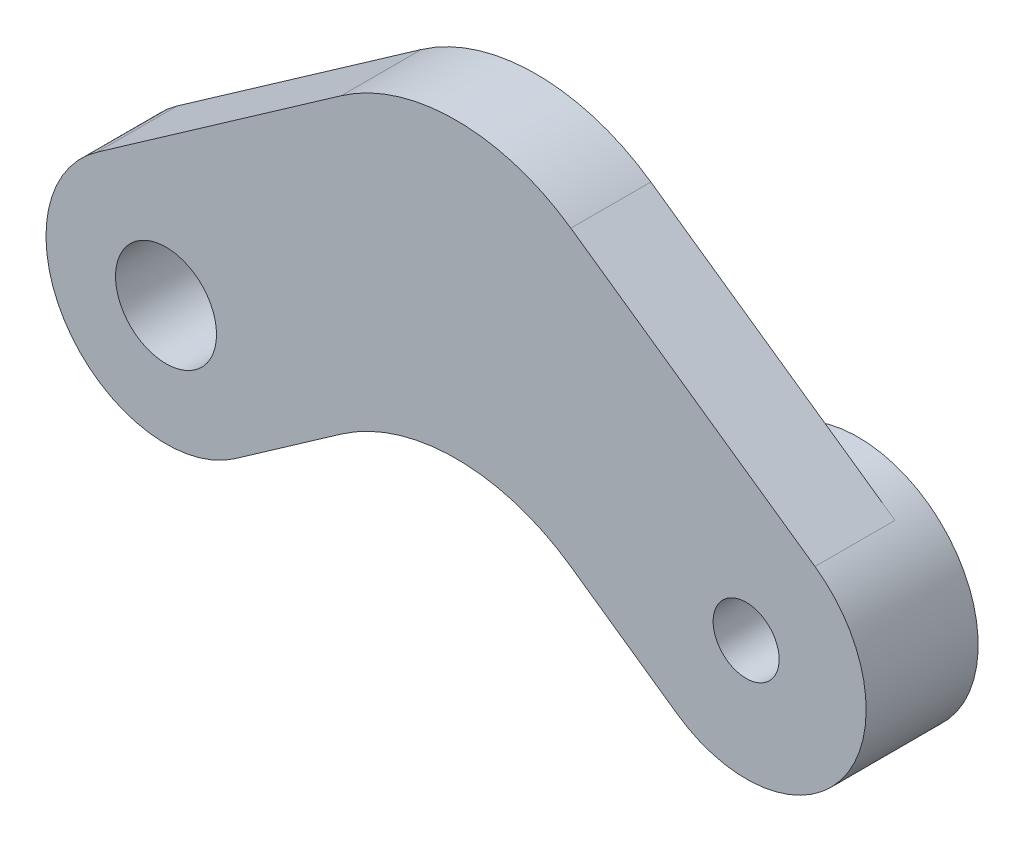
from build123d import *

# Parameters (mm, degrees)
BOSS_EXTRUDE1_DEPTH = 4
SKETCH2_R           = 2.525
CUT_EXTRUDE1_DEPTH  = 5
BOSS_EXTRUDE2_START = 1.6
SKETCH7_R           = 6
BOSS_EXTRUDE2_DEPTH = 1.6
M4_TAPPED_HOLE1_D   = 3.3
FILLET1_R           = 10


with BuildPart() as part:
    # Sketch1 → Boss-Extrude1 (new body)
    with BuildSketch(Plane.XY):
        with BuildLine():
            Line((3.441458618, -4.914912266), (14.5, 2.828361771))
            Line((14.5, 2.828361771), (25.558541382, -4.914912266))
            ThreePointArc((25.558541382, -4.914912266), (33.914912266, -3.441458618), (32.441458618, 4.914912266))
            Line((32.441458618, 4.914912266), (14.5, 17.477656837))
            Line((14.5, 17.477656837), (-3.441458618, 4.914912266))
            ThreePointArc((-3.441458618, 4.914912266), (-4.914912266, -3.441458618), (3.441458618, -4.914912266))
        make_face()
    extrude(amount=BOSS_EXTRUDE1_DEPTH)

    # Sketch2 → Cut-Extrude1 (cut)
    with BuildSketch(Plane.XY.offset(4)):
        Circle(SKETCH2_R)
    extrude(amount=-CUT_EXTRUDE1_DEPTH, mode=Mode.SUBTRACT)

    # Sketch7 → Boss-Extrude2 (add)
    with BuildSketch(Plane(origin=(0, 0, 0), x_dir=(-1, 0, 0), z_dir=(0, 0, -1)).offset(BOSS_EXTRUDE2_START)):
        with Locations((-29, 0)):
            Circle(SKETCH7_R)
    extrude(amount=-BOSS_EXTRUDE2_DEPTH)

    # M4 Tapped Hole1 (through all)
    with Locations(Plane.XY.offset(4)):
        with Locations((29, 0)):
            Hole(M4_TAPPED_HOLE1_D / 2)

    # Fillet1
    fillet1_edges = [part.edges().sort_by_distance(p)[0] for p in [
        (14.5, 17.477656837, 2),
        (14.5, 2.828361771, 2),
    ]]
    fillet(fillet1_edges, radius=FILLET1_R)


solid = part.part
